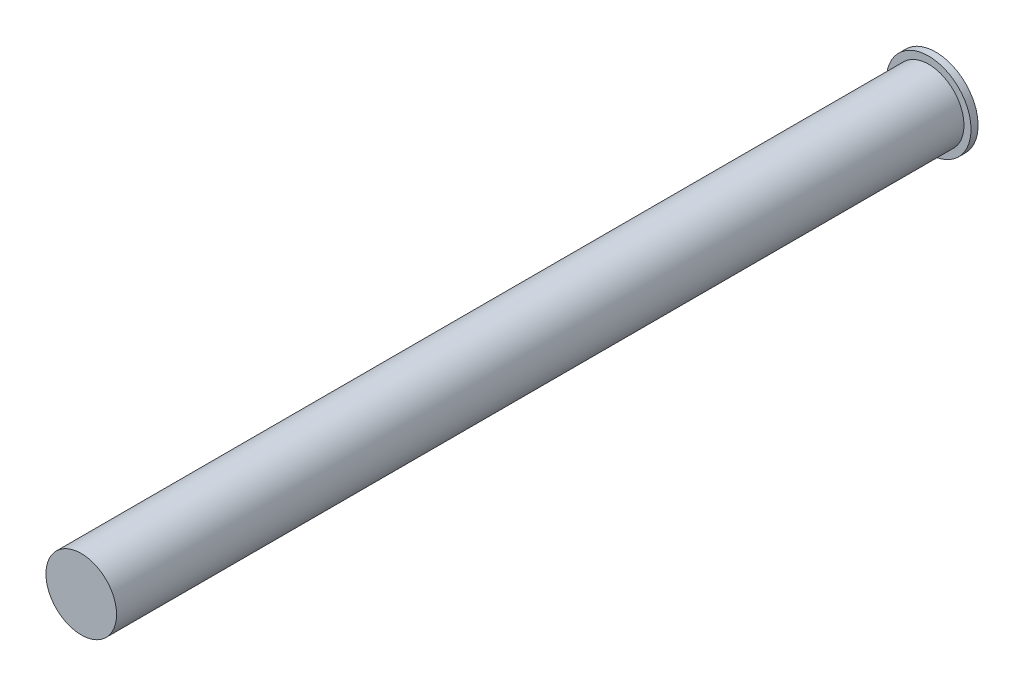
from build123d import *

# Parameters (mm, degrees)
SKETCH_1_R      = 5
EXTRUDE_1_DEPTH = 120
SKETCH_2_R      = 6
EXTRUDE_2_DEPTH = 1


with BuildPart() as part:
    # 草图1 → 凸台-拉伸1 (new body)
    with BuildSketch(Plane.XY):
        Circle(SKETCH_1_R)
    extrude(amount=EXTRUDE_1_DEPTH)

    # 草图2 → 凸台-拉伸2 (add)
    with BuildSketch(Plane(origin=(0, 0, 0), x_dir=(-1, 0, 0), z_dir=(0, 0, -1))):
        Circle(SKETCH_2_R)
    extrude(amount=EXTRUDE_2_DEPTH)


solid = part.part
